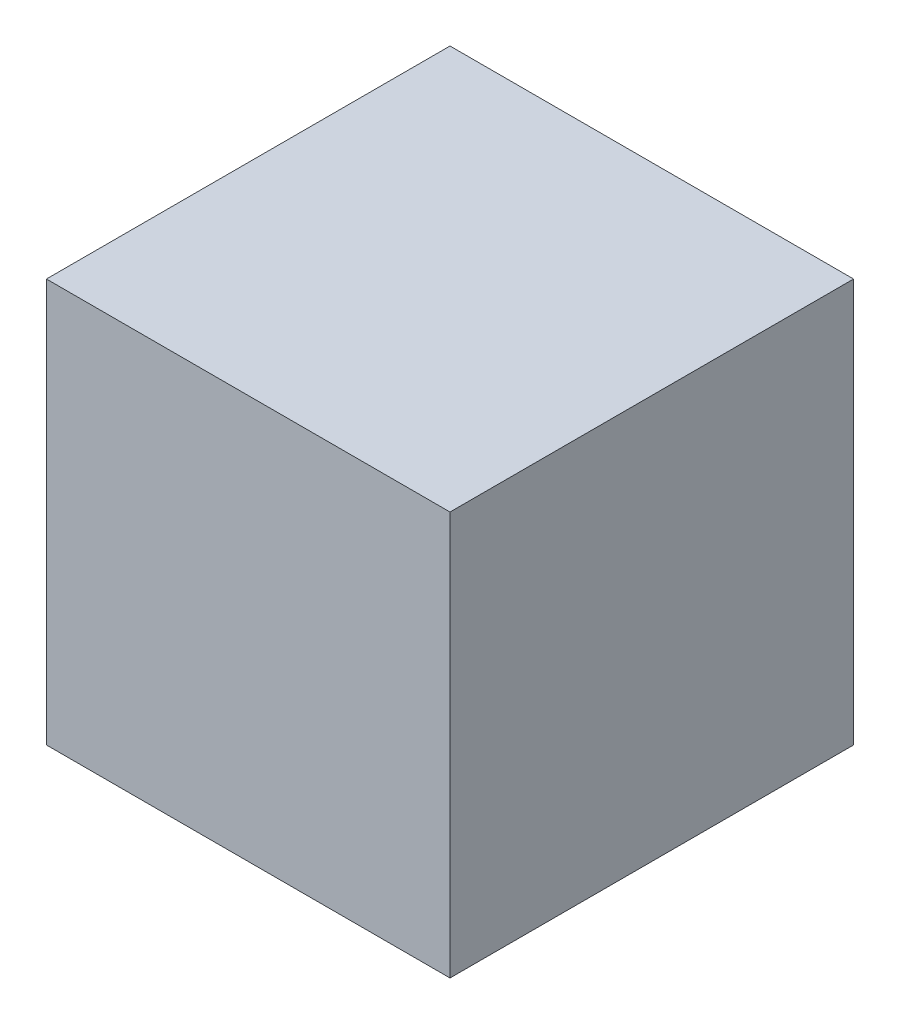
from build123d import *

# Parameters (mm, degrees)
SKETCH_1_W      = 80
SKETCH_1_H      = 80
EXTRUDE_1_DEPTH = 80


with BuildPart() as part:
    # 草图1 → 凸台-拉伸1 (new body)
    with BuildSketch(Plane.XY):
        Rectangle(SKETCH_1_W, SKETCH_1_H)
    extrude(amount=EXTRUDE_1_DEPTH)


solid = part.part
